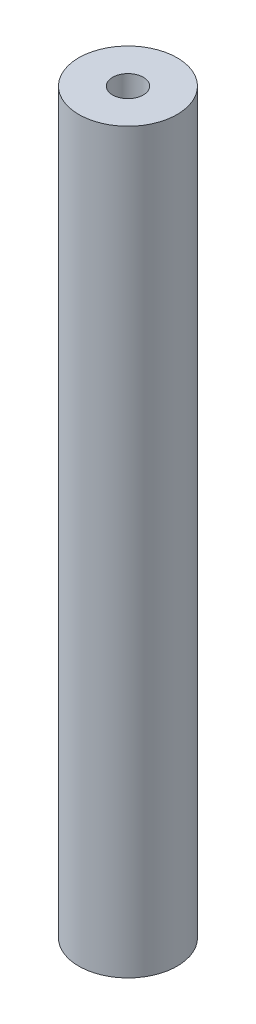
SolidWorks part; units mm, degrees
material "Zoltek Panex 33"
ref_plane "前视基准面" through (0, 0, 0) normal (0, 0, 1) x (1, 0, 0)
ref_plane "上视基准面" through (0, 0, 0) normal (0, 1, 0) x (1, 0, 0)
ref_plane "右视基准面" through (0, 0, 0) normal (1, 0, 0) x (0, 0, -1)
other "Configuration Table"
sketch "草图1" plane through (0, 0, 0) normal (0, 0, 1) x (1, 0, 0)
  line L0 (0, 60) -> (0, -60)
  point P4 (0, 0)
  dimension "D1" = 120
revolve "旋转-薄壁1" add sketch "草图1" angle 360 about L0 wall 8
hole_wizard "M6 螺纹孔的螺纹孔钻头1" positions "草图4" profile "草图5" hole size "M6" standard "GB"
sketch "草图4" plane through (0, 60, 0) normal (0, 1, 0) x (1, 0, 0)
  point P0 (0, 0)
sketch "草图5" plane through (0, 60, 0) normal (1, 0, 0) x (0, 0, 1)
  line L0 (0, 0) -> (0, 13.5022)
  line L1 (0, 13.5022) -> (2.5, 12)
  line L2 (2.5, 12) -> (2.5, 0)
  line L5 (2.5, 0) -> (0, 0)
  line L10 (0, 13.5022) -> (-2.5, 12) construction
  line L11 (0, -6.35) -> (0, 107.95) construction
  dimension "孔直径" = 5
  dimension "孔深度" = 12
  dimension "导头角度" = 118
hole_wizard "M6 螺纹孔的螺纹孔钻头2" positions "草图6" profile "草图7" hole size "M6" standard "GB"
sketch "草图6" plane through (0, -60, 0) normal (0, -1, 0) x (-1, 0, 0)
  point P0 (0, 0)
sketch "草图7" plane through (0, -60, 0) normal (1, 0, 0) x (0, 0, -1)
  line L0 (0, 0) -> (0, 13.5022)
  line L1 (0, 13.5022) -> (2.5, 12)
  line L2 (2.5, 12) -> (2.5, 0)
  line L5 (2.5, 0) -> (0, 0)
  line L10 (0, 13.5022) -> (-2.5, 12) construction
  line L11 (0, -6.35) -> (0, 107.95) construction
  dimension "孔直径" = 5
  dimension "孔深度" = 12
  dimension "导头角度" = 118
